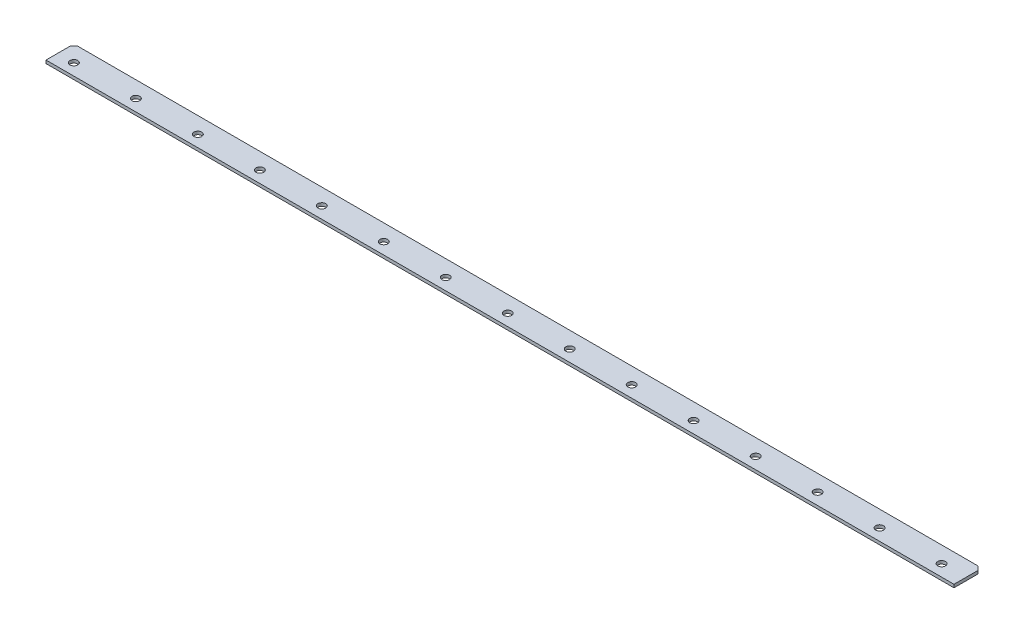
from build123d import *

# Parameters (mm, degrees)
SKETCH_1_W              = 1172
SKETCH_1_H              = 36
EXTRUDE_1_DEPTH         = 4
CHAMFER_1_SIZE          = 5
HOLE_WIZARD_10_0_10_1_D = 10
PATTERN_LINEAR_1_COUNT  = 15
PATTERN_LINEAR_1_PITCH  = 80


with BuildPart() as part:
    # 草图1 → 凸台-拉伸1 (new body)
    with BuildSketch(Plane(origin=(0, 0, 0), x_dir=(1, 0, 0), z_dir=(0, 1, 0))):
        with Locations((-586, -18)):
            Rectangle(SKETCH_1_W, SKETCH_1_H)
    extrude(amount=EXTRUDE_1_DEPTH)

    # 倒角1
    chamfer_1_edges = [part.edges().sort_by_distance(p)[0] for p in [
        (-1172, 2, 0),
        (0, 2, 0),
    ]]
    chamfer(chamfer_1_edges, length=CHAMFER_1_SIZE)

    # Ø10.0 (10) 直径孔1 (through all)
    with Locations(Plane(origin=(0, 4, 0), x_dir=(-1, 0, 0), z_dir=(0, 1, 0))):
        with Locations((1151, 21)):
            hole_wizard_10_0_10_1 = Hole(HOLE_WIZARD_10_0_10_1_D / 2)

    # 阵列(线性)1: Ø10.0 (10) 直径孔1 ×15
    with Locations(*[(i * PATTERN_LINEAR_1_PITCH, 0, 0) for i in range(1, PATTERN_LINEAR_1_COUNT)]):
        add(hole_wizard_10_0_10_1, mode=Mode.SUBTRACT)


solid = part.part
